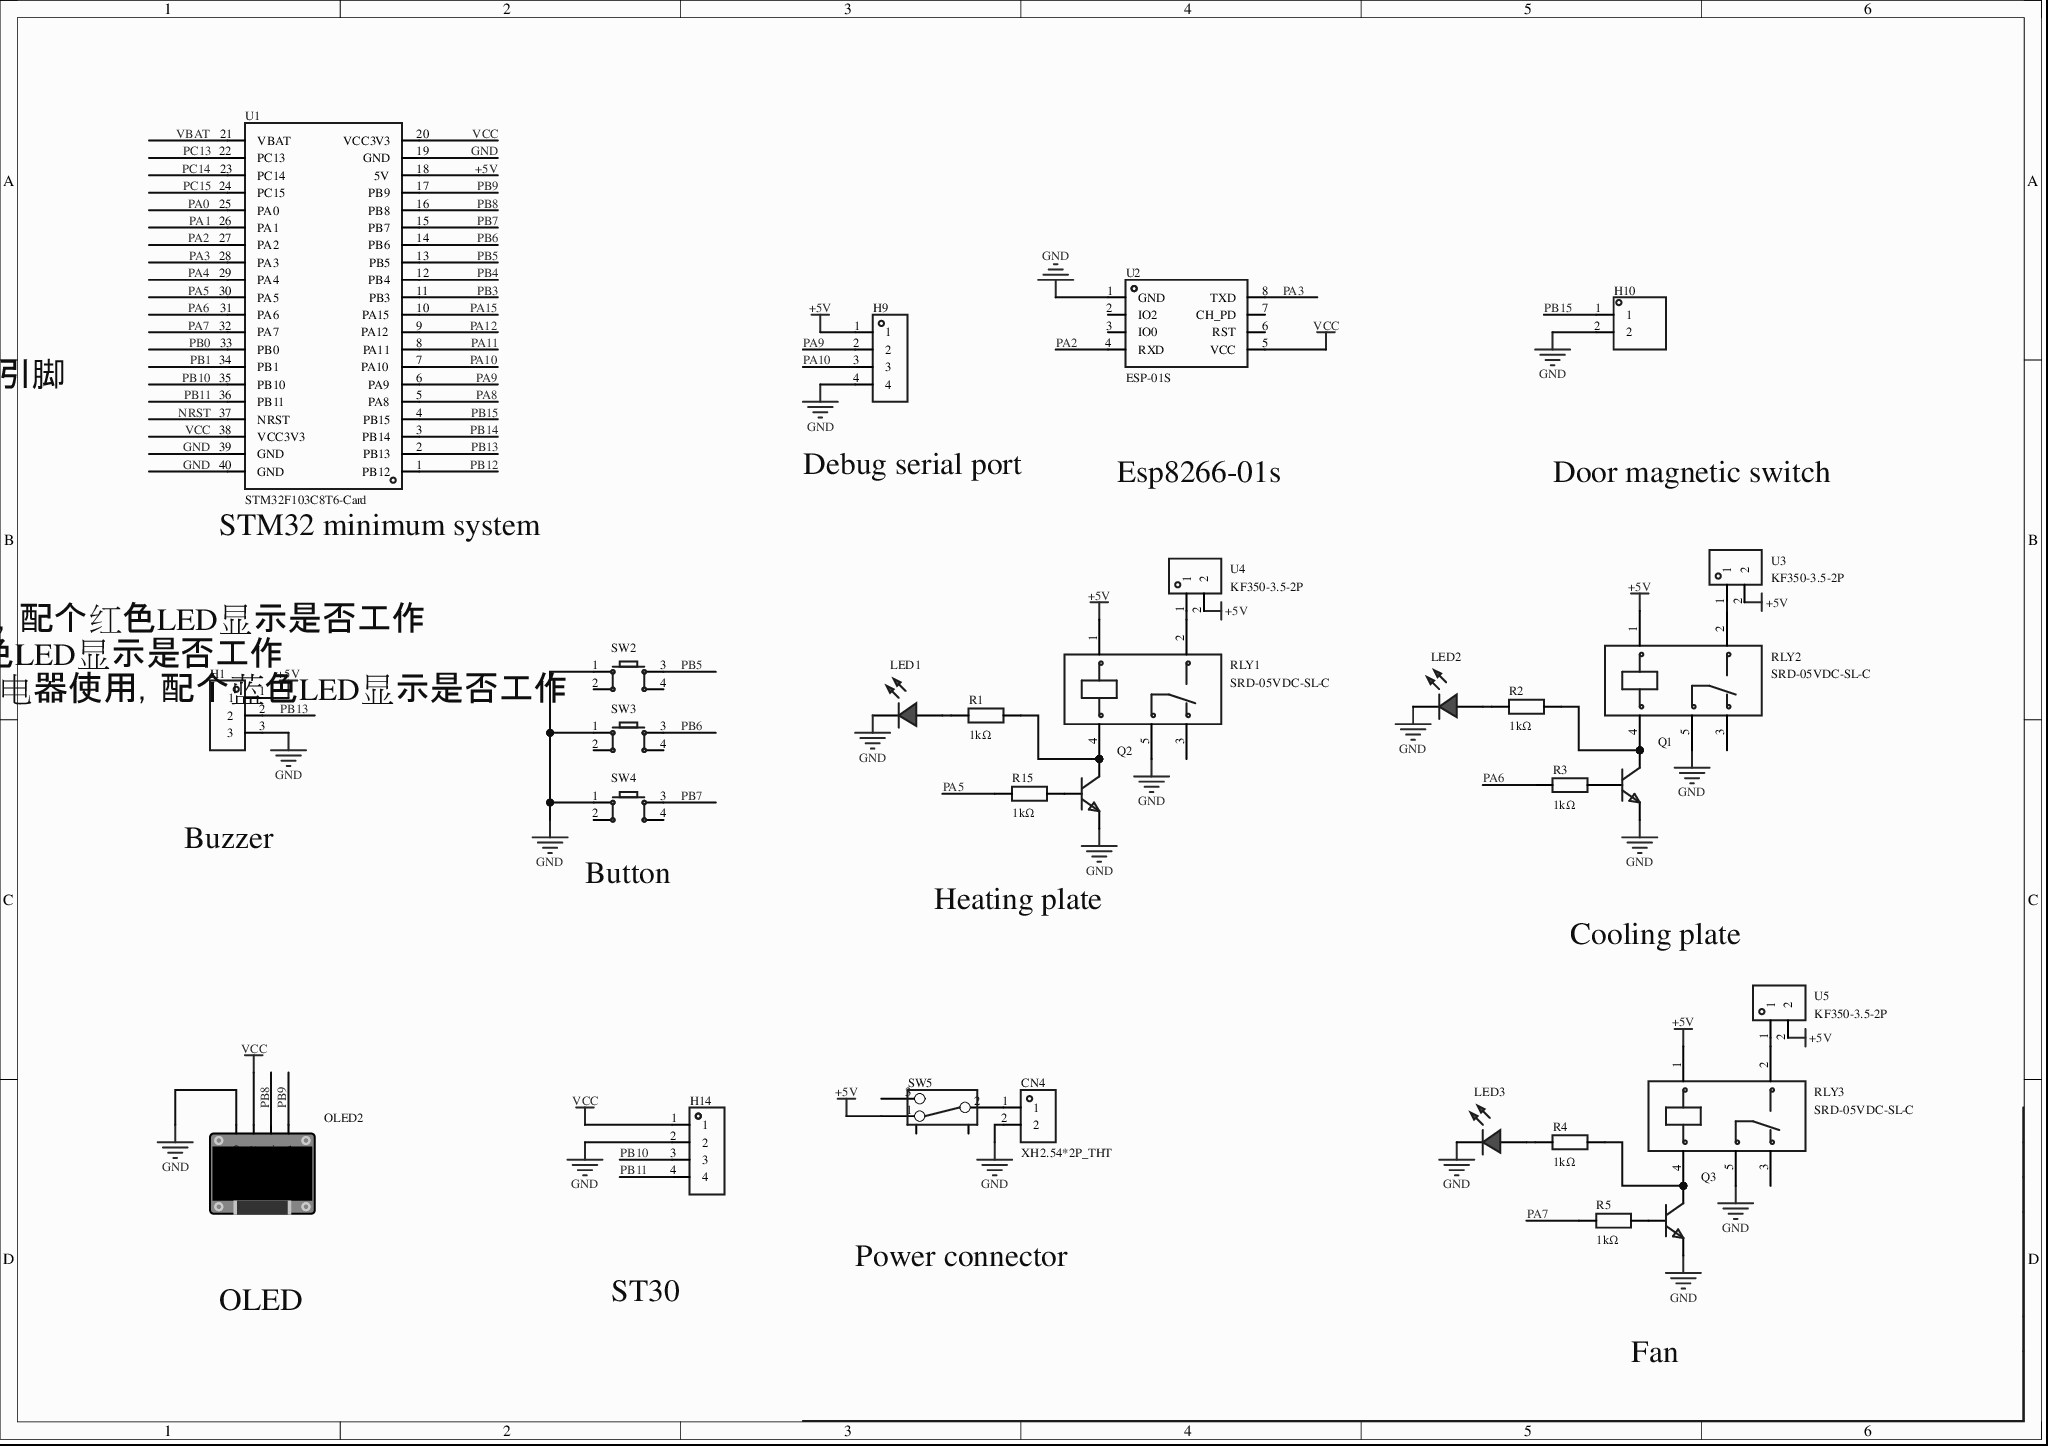
[diagram p0: MISC51783-3.schdoc]
# Altium project MISC51783-2.PrjPcb
1 sheet, 30 parts. Net scope: global (net labels, ports and power ports of the same name join across sheets).
Board file: MISC51783.pcbdoc

## Sheet MISC51783-3.schdoc
size 297 x 209 mm; Version: V1.0; @Project Name: MISC51783; @Page Count: 1; @Update Date: 2026-04-27; @Create Date: 2026-04-27; @Schematic Name: MISC51783; @Page No: 1; @Create Time: 23:22:16; @Update Time: 17:32:40; @Board Name: MISC51783

### Parts
CN4  XH2.54*2P_THT  [CONN-TH_2P-P2.50-XH2.54-2P]
H1  (no value)  [HDR-TH_3P-P2.54-V-F]
H9  (no value)  [HDR-TH_4P-P2.54-V-M]
H10  (no value)  [HDR-TH_2P-P2.54-V-M-1]
H14  (no value)  [HDR-TH_4P-P2.54-V-F]
LED1  (no value)  [LED_TH-3mm]
LED2  (no value)  [LED_TH-3mm]
LED3  (no value)  [LED_TH-3mm]
OLED2  (no value)  [0.96OLED_4P]
Q1  (no value)  [S8050_TO_92]
Q2  (no value)  [S8050_TO_92]
Q3  (no value)  [S8050_TO_92]
R1  1kΩ  [Res_1/4W]
R2  1kΩ  [Res_1/4W]
R3  1kΩ  [Res_1/4W]
R4  1kΩ  [Res_1/4W]
R5  1kΩ  [Res_1/4W]
R15  1kΩ  [Res_1/4W]
RLY1  SRD-05VDC-SL-C  [RELAY-TH_SRD-XXVDC-XL-C]
RLY2  SRD-05VDC-SL-C  [RELAY-TH_SRD-XXVDC-XL-C]
RLY3  SRD-05VDC-SL-C  [RELAY-TH_SRD-XXVDC-XL-C]
SW2  (no value)  [SW-TH_4P-L6.0-W6.0-P4.50-LS6.5]
SW3  (no value)  [SW-TH_4P-L6.0-W6.0-P4.50-LS6.5]
SW4  (no value)  [SW-TH_4P-L6.0-W6.0-P4.50-LS6.5]
SW5  (no value)  [拨动开关]
U1  STM32F103C8T6-Card  [CONN-TH_L53.3-W22.9_STM32F103C8T6-CARD]
U2  ESP-01S  [WIFIM-TH_ESP-01S]
U3  KF350-3.5-2P  [CONN-TH_P3.50_KF350-3.5-2P]
U4  KF350-3.5-2P  [CONN-TH_P3.50_KF350-3.5-2P]
U5  KF350-3.5-2P  [CONN-TH_P3.50_KF350-3.5-2P]

### Nets
+5V: H1.1 H9.1 RLY1.1 RLY2.1 RLY3.1 SW5.1 U1.18(5V) U3.2 U4.2 U5.2
GND: CN4.2 H1.3 H9.4 H10.2 H14.2 LED1.2(A) LED2.2(A) LED3.2(A) OLED2.1(GND) Q1.1(E) Q2.1(E) Q3.1(E) RLY1.5 RLY2.5 RLY3.5 SW2.1 SW3.1 SW4.1 U1.19(GND) U1.39(GND) U1.40(GND) U2.1(GND)
VCC: H14.1 OLED2.2(VCC) U1.20(VCC3V3) U1.38(VCC3V3) U2.5(VCC)
NRST: U1.37(NRST)
PA0: U1.25(PA0)
PA1: U1.26(PA1)
PA2: U1.27(PA2) U2.4(RXD)
PA3: U1.28(PA3) U2.8(TXD)
PA4: U1.29(PA4)
PA5: R15.1 U1.30(PA5)
PA6: R3.1 U1.31(PA6)
PA7: R5.1 U1.32(PA7)
PA8: U1.5(PA8)
PA9: H9.2 U1.6(PA9)
PA10: H9.3 U1.7(PA10)
PA11: U1.8(PA11)
PA12: U1.9(PA12)
PA15: U1.10(PA15)
PB0: U1.33(PB0)
PB1: U1.34(PB1)
PB3: U1.11(PB3)
PB4: U1.12(PB4)
PB5: SW2.3 U1.13(PB5)
PB6: SW3.3 U1.14(PB6)
PB7: SW4.3 U1.15(PB7)
PB8: OLED2.3(SCL) U1.16(PB8)
PB9: OLED2.4(SDA) U1.17(PB9)
PB10: H14.3 U1.35(PB10)
PB11: H14.4 U1.36(PB11)
PB12: U1.1(PB12)
PB13: H1.2 U1.2(PB13)
PB14: U1.3(PB14)
PB15: H10.1 U1.4(PB15)
PC13: U1.22(PC13)
PC14: U1.23(PC14)
PC15: U1.24(PC15)
VBAT: U1.21(VBAT)
NetCN4_1: CN4.1 SW5.2
NetLED1_1: LED1.1(C) R1.1
NetLED2_1: LED2.1(C) R2.1
NetLED3_1: LED3.1(C) R4.1
NetQ1_2: Q1.2(B) R3.2
NetQ1_3: Q1.3(C) R2.2 RLY2.4
NetQ2_2: Q2.2(B) R15.2
NetQ2_3: Q2.3(C) R1.2 RLY1.4
NetQ3_2: Q3.2(B) R5.2
NetQ3_3: Q3.3(C) R4.2 RLY3.4
NetRLY1_2: RLY1.2 U4.1
NetRLY2_2: RLY2.2 U3.1
NetRLY3_2: RLY3.2 U5.1

Not connected (* = marked no-connect by the designer): RLY1 3; RLY2 3; RLY3 3; SW2 2 4; SW3 2 4; SW4 2 4; SW5 3 4 5; U2 2(IO2)* 3(IO0)* 6(RST)* 7(CH_PD)*

### Notes on the sheet
- 串口：
  串口1：	TX-PA9		RX-PA10		调试串口
  串口2：	TX-PA2		RX-PA3			此为esp8266通信引脚
  GPIO:
  门磁开关：			PB15
  蜂鸣器：			PB13		低电位响
  三个按键：			PB5,6,7		并排连接
  PTC加热片：		PA5			配合继电器使用，配个红色LED显示是否工作
  TEC1-04903/制冷片：PA6			配合继电器使用，配个白色LED显示是否工作
  微型风扇：			PA7			配合继电器使用，配个蓝色LED显示是否工作
  IIC:
  0.96英寸OLED显示屏	PB8，PB9
  SHT30：					PB10,PB11
  供电：我没搞，你看着来
- (near H9) Debug serial port
- Esp8266-01s
- Door magnetic switch
- (near U1) STM32 minimum system
- Buzzer
- (near SW4) Button
- Heating plate
- Cooling plate
- ST30
- Power connector
- OLED
- Fan

### Library data of the parts
CN4 = XH2.54*2P_直插: 3D Model: 325c595e30db4df8abe76612dd40b0fa0819f05c4eef4c71ace90d822a990e87; 3D Model Transform: 295.275,228.346,0,180,0,0,-0.002,-20.079,-137.795; AddInBom: yes; Device: XH2.54*2P_THT; Symbol: XH2.54*2P_THT; LCSC Part Name: XH2.54*2P_直插; Supplier Part: C9900008615; Manufacturer Part: XH2.54*2P_直插; Supplier Footprint: XH2.54_2P; JLCPCB Part Class: Extended Part; Supplier: LCSC; FootprintName: CONN-TH_2P-P2.50-XH2.54-2P; ConvertToPcb: yes; ModelName: CONN-TH_2P-P2.50-XH2.54-2P
H1 = HDR-F_2.54_1x3P: Symbol: PM254V-11-03-H85; 3D Model: f3b3cc5aae9641bf9e56fc160cef875b; 3D Model Transform: 299.9994,100,0,0,0,0,0,0,-118.11; ConvertToPcb: yes; ModelName: HDR2.54-F-LI-1X3P; Device: HDR-F_2.54_1x3P; Supplier Part: C541850; Supplier Footprint: 插件; FootprintName: HDR-TH_3P-P2.54-V-F; AddInBom: yes
H9 = HDR-M_2.54_1x4P: Symbol: PZ254V-11-04P; 3D Model: 112f4d05e8d64e99ab9a333894bea4f90819f05c4eef4c71ace90d822a990e87; 3D Model Transform: 399.999,104.7242,0,0,0,0,0,0,-118.11; ConvertToPcb: yes; ModelName: HDR-TH_4P-P2.54-M-LI-1X4P; Device: HDR-M_2.54_1x4P; Supplier Part: C492403; Supplier Footprint: 插件; AddInBom: yes; FootprintName: HDR-TH_4P-P2.54-V-M
H10 = HDR-M_2.54_1x2P: Symbol: 210S-1*2P L=11.6MMGold-plated black; ConvertToPcb: yes; ModelId: 79b2e9f2d70a4d68a1b7098f27c6d4c50819f05c4eef4c71ace90d822a990e87; ModelName: HDR-M-2.54_1x2; ModelTransform: 200,100,0,0,0,0,0,0,-118.11; Device: HDR-M_2.54_1x2P; AddInBom: yes; SupplierPart: C124375; Supplier Footprint: 插件; FootprintName: HDR-TH_2P-P2.54-V-M-1
H14 = HDR-F_2.54_1x4P: Symbol: 2.54-1*4P female; ConvertToPcb: yes; ModelId: d187812051054f85879fcaa51a310d8e0819f05c4eef4c71ace90d822a990e87; ModelTransform: 419.6842,98.464,0,0,0,0,0,0,-118.11; Device: HDR-F_2.54_1x4P; AddInBom: yes; SupplierPart: C2718488; Supplier Footprint: 插件; FootprintName: HDR-TH_4P-P2.54-V-F; ModelName: HDR-TH_4P-P2.54-V-F
LED1-LED3 = LED_TH-R_3mm: 3D Model: a497c992633541038a38947cdc58012f0819f05c4eef4c71ace90d822a990e87; 3D Model Transform: 141.274,153.327,0,0,0,0,-5.984,0,-137.795; ConvertToPcb: yes; ModelName: LED-TH-3mm_R; Symbol: LED_TH-R; Device: LED_TH-R_3mm; Supplier Footprint: 插件; AddInBom: yes; FootprintName: LED_TH-3mm
OLED2 = 0.96OLED模块_4P: Symbol: 0.96OLED module_4P; ConvertToPcb: yes; ModelId: 79c000fdb68d45a296c2e9bedf4f9055; ModelTransform: 1393.69792,1318.895,0,0,0,0,0,-560.079,-137.795; Device: 0.96OLED module_4P; AddInBom: yes; FootprintName: 0.96OLED_4P; Supplier Footprint: 插件; ModelName: 0.96OLED_4P
Q1-Q3 = S8050_TO_NPN: 3D Model: aafe8e06f2154e7c93506efd0d6632dd; 3D Model Transform: 180.78,141.44,417.3,0,0,0,0,0,-200; ConvertToPcb: yes; ModelName: TO-92-3_L4.9-W3.7-P1.27-L; Symbol: S8050_TO_NPN; Device: S8050_TO_NPN; Supplier Footprint: TO-92; AddInBom: yes; FootprintName: S8050_TO_92
R1-R5 R15 = Res_AXIAL-1/8W: Symbol: Resistor; 3D Model: b2b5ae7ae4c642178fe0039925c86a3f0819f05c4eef4c71ace90d822a990e87; 3D Model Transform: 282.86,66.88,253.09,0,0,0,0,0,-191; ConvertToPcb: yes; ModelName: RES-TH_BD1.8-L3.2-P7.20-D0.4; Device: Res_AXIAL-1/8W; Supplier Footprint: 轴向引线; Value: 1kΩ; AddInBom: yes; FootprintName: Res_1/4W
RLY1-RLY3 = SRD-05VDC-SL-C: Coil voltage:5V;Contact form:One changeover:1C(SPDT);Contact rating(resistive load):-;Max switching voltage:250V@AC;Max switching current:15A;; Manufacturer: 松乐; 3D Model: d0eda9b8bf8746d18ae810ab88dc78e70819f05c4eef4c71ace90d822a990e87; 3D Model Transform: 755.904,622.4397,0,0,0,0,34.882,0,-118.11; Coil Voltage: 5V; Coil Rated Power: 360mW; Switching Current(Max): 15A; Coil Type: Non-polar, single coil; Coil Resistance: 70Ω; Contact Resistance: 100mΩ; Operate Time: 10ms; AddInBom: yes; ModelName: RELAY-TH_L19.2-W15.6-H15.8; Symbol: SRD-05VDC-SL-C; Device: SRD-05VDC-SL-C; LCSC Part Name: 蓝色 单组转换型继电器; Supplier Part: C35449; Manufacturer Part: SRD-05VDC-SL-C; Supplier Footprint: 插件,19.2x15.6mm; JLCPCB Part Class: Extended Part; Datasheet: https://item.szlcsc.com/datasheet/SRD-05VDC-SL-C/36422.html; Supplier: LCSC; Contact Form: One changeover:1C(SPDT); Number of Pins: 5; Contact Rating: -; Switching Voltage(Max): 250V@AC; Release Time: 10ms; ConvertToPcb: yes; FootprintName: RELAY-TH_SRD-XXVDC-XL-C
SW2-SW4 = Key_TH_6x6x6: Contact current:50mA;Rated voltage(DC):12V;Insulation resistance:100MΩ;Circuit:SPST;Mounting:through-hole;Button shape:round button;Button/cap colour:black;Actuating force:260gf@±30gf;Operating temperature:-25℃~+70℃;Pin style:PC pin;Switch length:6mm;Switch width:6mm;Switch height:6mm;With bracket:no;; Symbol: Tactile button; AddInBom: yes; ModelId: 20eee248bc684ccd8cbdbb1d0d91ec6f0819f05c4eef4c71ace90d822a990e87; ModelName: SW-TH_4P-L6.0-W6.0-H5.0-LS6.5-P4.50; ModelTransform: 236.22,323.03,0,90,0,0,0,0,-137.795; Device: Key_TH_6x6x6; FootprintName: SW-TH_4P-L6.0-W6.0-P4.50-LS6.5; ConvertToPcb: yes; Supplier Footprint: 插件
SW5 = 拨动开关_正: Device: Toggle switch_pos; Symbol: Toggle switch; ConvertToPcb: yes; ModelId: 4321fe59a4074cbfb4989553f297c68f0819f05c4eef4c71ace90d822a990e87; ModelName: SW-TH_SS-12D02-VG4; ModelTransform: 370.09,208.7,472.35,0,0,0,0,0,-110; FootprintName: Toggle switch; AddInBom: yes; Supplier Footprint: 插件
U1 = STM32F103C8T6-Card: AddInBom: yes; Device: STM32F103C8T6-Card; Symbol: STM32F103C8T6-CARD; FootprintName: CONN-TH_L53.3-W22.9_STM32F103C8T6-CARD; LCSC Part Name: STM32F103C8T6-Card; SupplierPart: C9900077949; ManufacturerPart: STM32F103C8T6-Card; Supplier Footprint: 插件; Supplier: LCSC; ConvertToPcb: yes
U2 = ESP-01S_C111009: 3D Model: eb7175da78ae48b3b1568cfe3027405f0819f05c4eef4c71ace90d822a990e87; 3D Model Transform: 582.676,976.37608,0,0,0,0,0,388.346,-118.11; AddInBom: yes; Symbol: ESP-01S; Device: ESP-01S_C111009; LCSC Part Name: ESP-01S; Supplier Part: C111009; Manufacturer Part: ESP-01S; Supplier Footprint: -; JLCPCB Part Class: Extended Part; Supplier: LCSC; ConvertToPcb: yes; FootprintName: WIFIM-TH_ESP-01S; ModelName: WIFIM-TH_ESP-01S
U3-U5 = KF350-3.5-2P: Structure:1x2P;Pitch:3.5mm;Colour:green;Mounting:through-hole;Rated current:10A;Rated voltage:300V;Rows:1;Wire gauge - AWG:18~24;Wire gauge - mm2:0.75;Pins per row:2;Operating temperature range:-40℃~+105℃;; Manufacturer: KEFA(科发); 3D Model: b1d1e83e7d6a49aab33370f0163c64ca0819f05c4eef4c71ace90d822a990e87; 3D Model Transform: 314.96,271.653,0,0,0,0,0,1.968,-133.858; Structure: 1x2P; Pitch: 3.5mm; Current Rating (Max): 10A; Voltage Rating (Max): 300V; Wire Gauge - AWG: 18~24; Wire Gauge - mm2: 0.75; Number of PINs Per Row: 2; AddInBom: yes; Symbol: KF350-3.5-2P; Device: KF350-3.5-2P; LCSC Part Name: 3.5mm 1x2P 排数:1 每排P数:2 直插; Supplier Part: C474892; Manufacturer Part: KF350-3.5-2P; Supplier Footprint: 插件,P=3.5mm; JLCPCB Part Class: Extended Part; Datasheet: https://atta.szlcsc.com/upload/public/pdf/source/20230317/986DB56DD49619EA586AA8816AA9D164.pdf; Supplier: LCSC; Color: Green; Mounting Style: Through-hole; Number of Pins: 2P; Number of Rows: 1; Operating Temperature Range: -40℃~+105℃; ConvertToPcb: yes; FootprintName: CONN-TH_P3.50_KF350-3.5-2P; ModelName: CONN-TH_P3.50_KF350-3.5-2P